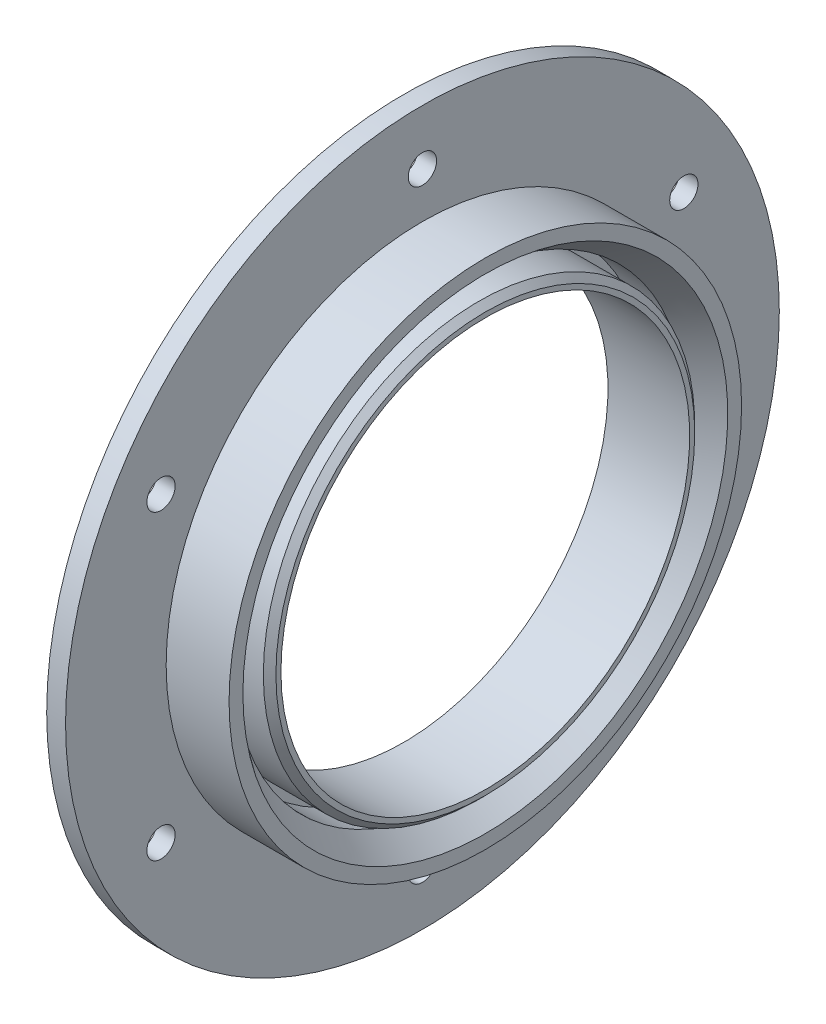
SolidWorks part; units mm, degrees
material "ABS"
ref_plane "Front Plane" through (0, 0, 0) normal (0, 0, 1) x (1, 0, 0)
ref_plane "Top Plane" through (0, 0, 0) normal (0, 1, 0) x (1, 0, 0)
ref_plane "Right Plane" through (0, 0, 0) normal (1, 0, 0) x (0, 0, -1)
sketch "Sketch1" plane through (0, 0, 0) normal (0, 0, 1) x (1, 0, 0)
  line L0 (0, 32.5) -> (13, 32.5)
  line L1 (13, 32.5) -> (13, 34.3)
  line L2 (13, 34.3) -> (3, 34.3)
  line L3 (3, 34.3) -> (3, 35.75)
  line L4 (3, 35.75) -> (13, 35.75)
  line L5 (13, 35.75) -> (13, 40.75)
  line L6 (13, 40.75) -> (3, 40.75)
  line L7 (3, 40.75) -> (3, 56.75)
  line L8 (3, 56.75) -> (0, 56.75)
  line L9 (0, 56.75) -> (0, 32.5)
  line L10 (0, 0) -> (19.9956, 0) construction
  dimension "D1" = 3
  dimension "D2" = 35.75
  dimension "D3" = 34.3
  dimension "D4" = 10
  dimension "D5" = 32.5
  dimension "D6" = 5
  dimension "D7" = 16
revolve "Revolve1" add sketch "Sketch1" angle 360 about L10
chamfer "Chamfer1" distance 4 angle 35 1 edges at (13, 0, 35.75)
chamfer "Chamfer2" distance 1 angle 45 1 edges at (13, 0, 34.3)
sketch "Sketch2" plane through (3, 0, 0) normal (1, 0, 0) x (0, 0, -1)
  circle A0 centre (0, 48) radius 2.25
  dimension "D1" = 48
  dimension "D2" = 4.5
extrude "Cut-Extrude1" cut sketch "Sketch2" against normal blind 10
pattern_circular "CirPattern1" count 6 over 360 about axis through (0, 0, 0) along (1, 0, 0) of "Cut-Extrude1"
